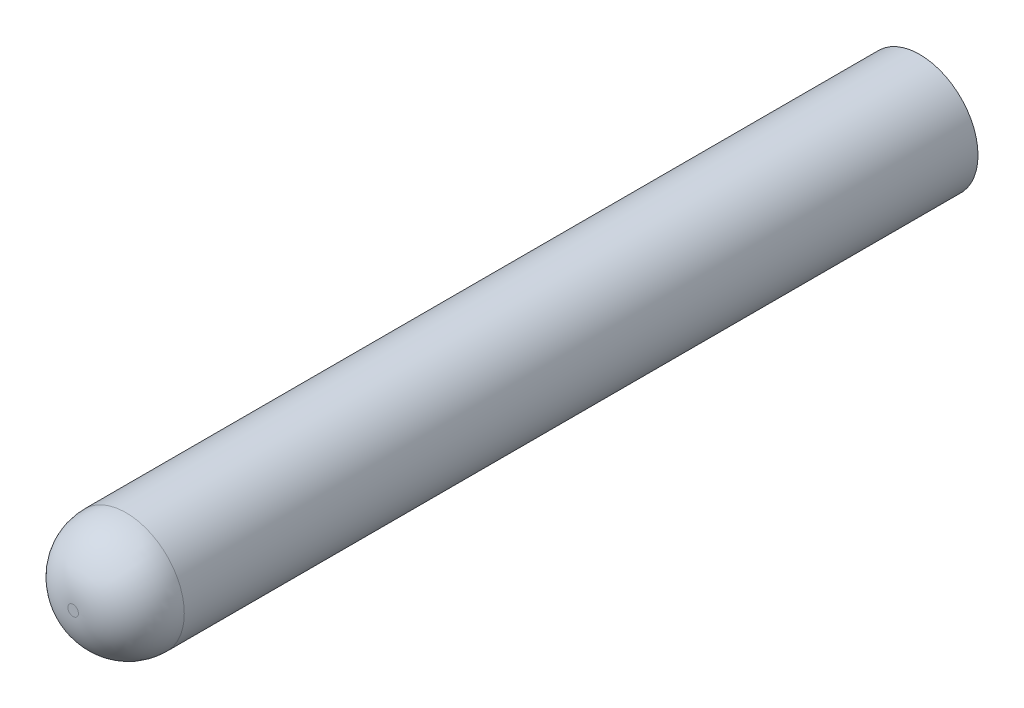
from build123d import *

# Parameters (mm, degrees)
SKETCH1_R           = 1.1
BOSS_EXTRUDE1_DEPTH = 16
FILLET1_R           = 1


with BuildPart() as part:
    # Sketch1 → Boss-Extrude1 (new body)
    with BuildSketch(Plane.XY):
        Circle(SKETCH1_R)
    extrude(amount=BOSS_EXTRUDE1_DEPTH)

    # Fillet1
    fillet1_edges = [part.edges().sort_by_distance(p)[0] for p in [
        (-1.1, 0, 16),
    ]]
    fillet(fillet1_edges, radius=FILLET1_R)


solid = part.part
